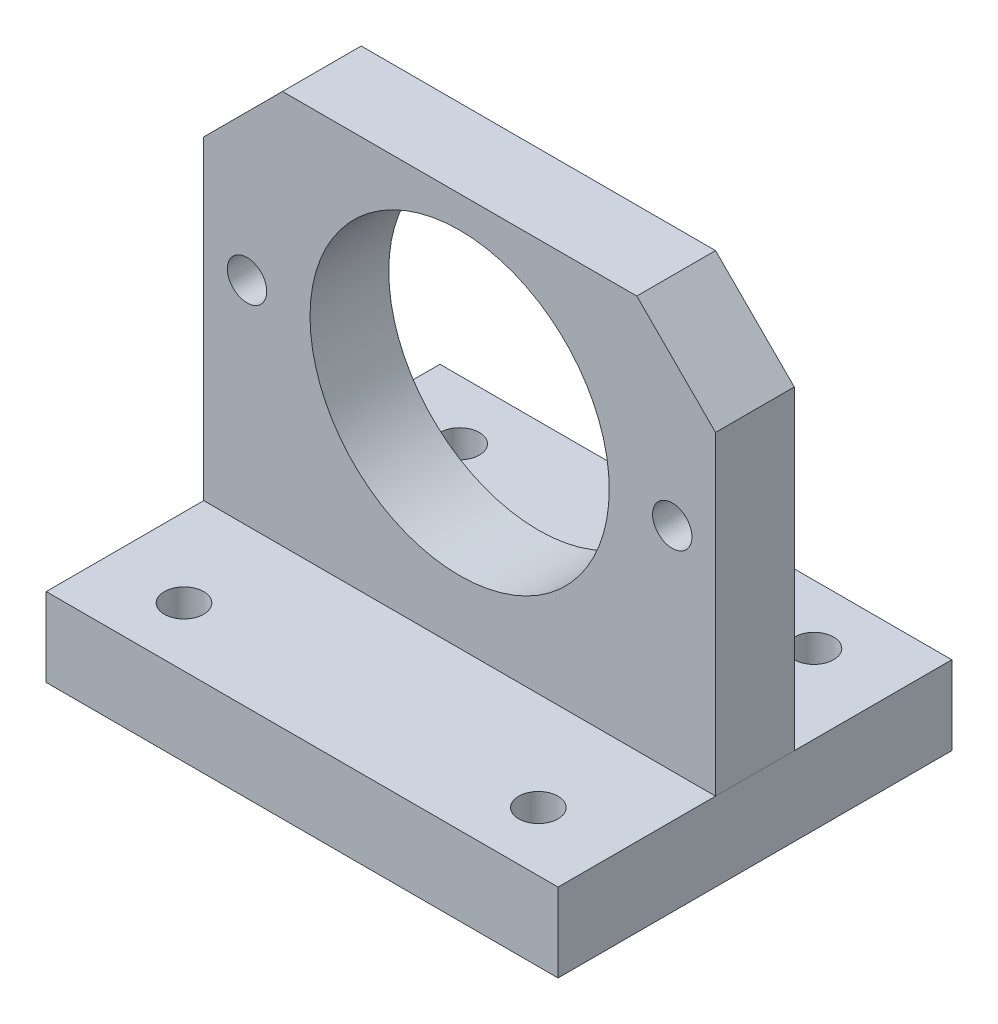
SolidWorks part; units mm, degrees
ref_plane "Front Plane" through (0, 0, 0) normal (0, 0, 1) x (1, 0, 0)
ref_plane "Top Plane" through (0, 0, 0) normal (0, 1, 0) x (1, 0, 0)
ref_plane "Right Plane" through (0, 0, 0) normal (1, 0, 0) x (0, 0, -1)
sketch "Sketch1" plane through (0, 0, 0) normal (0, 1, 0) x (1, 0, 0)
  line L1 (-32.5, 25) -> (32.5, 25)
  line L2 (-32.5, 25) -> (-32.5, -25)
  line L3 (-32.5, -25) -> (32.5, -25)
  line L4 (32.5, 25) -> (32.5, -25)
  line L5 (-32.5, 25) -> (32.5, -25) construction
  line L6 (-32.5, -25) -> (32.5, 25) construction
  point P0 (0, 0)
  dimension "D1" = 65
  dimension "D2" = 50
extrude "Boss-Extrude1" add sketch "Sketch1" along normal blind 10
sketch "Sketch2" plane through (0, 10, 0) normal (0, 1, 0) x (1, 0, 0)
  line L0 (32.5, -25) -> (32.5, 25) construction
  line L1 (-32.5, 5) -> (32.5, 5)
  line L2 (-32.5, 5) -> (-32.5, -5)
  line L3 (-32.5, -5) -> (32.5, -5)
  line L4 (32.5, 5) -> (32.5, -5)
  line L5 (-32.5, 5) -> (32.5, -5) construction
  line L6 (-32.5, -5) -> (32.5, 5) construction
  point P0 (0, 0)
  dimension "D1" = 10
extrude "Boss-Extrude2" add sketch "Sketch2" along normal blind 50 separate body
sketch "Sketch3" plane through (0, 0, 5) normal (0, 0, 1) x (1, 0, 0)
  line L0 (0, 0) -> (0, 60) construction
  line L1 (-32.5, 60) -> (32.5, 60) construction
  line L2 (-32.5, 0) -> (32.5, 0) construction
  circle A0 centre (0, 37) radius 19
  dimension "D1" = 38
  dimension "D2" = 37
extrude "Cut-Extrude1" cut sketch "Sketch3" against normal up to next (10 mm away)
chamfer "Chamfer1" distance 10 angle 45 2 edges at (32.5, 60, 0) (-32.5, 60, 0)
hole_wizard "M6 Tapped Hole2" positions "Sketch4" profile "Sketch5" tap size "M6" standard "GB" end condition through all
sketch "Sketch4" plane through (0, 10, 0) normal (0, 1, 0) x (1, 0, 0)
  line L1 (-22.5, 17.5) -> (22.5, 17.5) construction
  line L2 (-22.5, 17.5) -> (-22.5, -17.5) construction
  line L3 (-22.5, -17.5) -> (22.5, -17.5) construction
  line L4 (22.5, 17.5) -> (22.5, -17.5) construction
  line L5 (-22.5, 17.5) -> (22.5, -17.5) construction
  line L6 (-22.5, -17.5) -> (22.5, 17.5) construction
  point P2 (22.5, -17.5)
  point P125 (-22.5, 17.5)
  point P126 (-22.5, -17.5)
  point P127 (22.5, 17.5)
  dimension "D1" = 35
  dimension "D2" = 45
sketch "Sketch5" plane through (22.5, 10, 17.5) normal (1, 0, 0) x (0, 0, 1)
  line L0 (0, 0) -> (0, 10)
  line L1 (0, 10) -> (2.5, 10)
  line L2 (2.5, 10) -> (2.5, 0)
  line L5 (2.5, 0) -> (0, 0)
  line L11 (0, -6.35) -> (0, 107.95) construction
  dimension "通孔螺纹孔钻头直径" = 5
  dimension "通孔螺纹孔钻头深度" = 10
cosmetic thread "Cosmetic Thread3" parameters "D2"=6
cosmetic thread "Cosmetic Thread4" parameters "D2"=6
cosmetic thread "Cosmetic Thread5" parameters "D2"=6
cosmetic thread "Cosmetic Thread6" parameters "D2"=6
hole_wizard "M6 Tapped Hole1" positions "Sketch6" profile "Sketch7" tap size "M6" standard "GB" end condition up to next
sketch "Sketch6" plane through (0, 0, 5) normal (0, 0, 1) x (1, 0, 0)
  line L0 (-27, 37) -> (27, 37) construction
  circle A0 centre (0, 37) radius 27 construction
  point P5 (-27, 37)
  point P6 (27, 37)
  dimension "D1" = 54
sketch "Sketch7" plane through (-27, 37, 5) normal (1, 0, 0) x (0, -1, 0)
  line L0 (0, 0) -> (0, 10)
  line L1 (0, 10) -> (2.5, 10)
  line L2 (2.5, 10) -> (2.5, 0)
  line L5 (2.5, 0) -> (0, 0)
  line L11 (0, -6.35) -> (0, 107.95) construction
  dimension "通孔螺纹孔钻头直径" = 5
  dimension "通孔螺纹孔钻头深度" = 10
cosmetic thread "Cosmetic Thread1" parameters "D2"=6
cosmetic thread "Cosmetic Thread2" parameters "D2"=6
